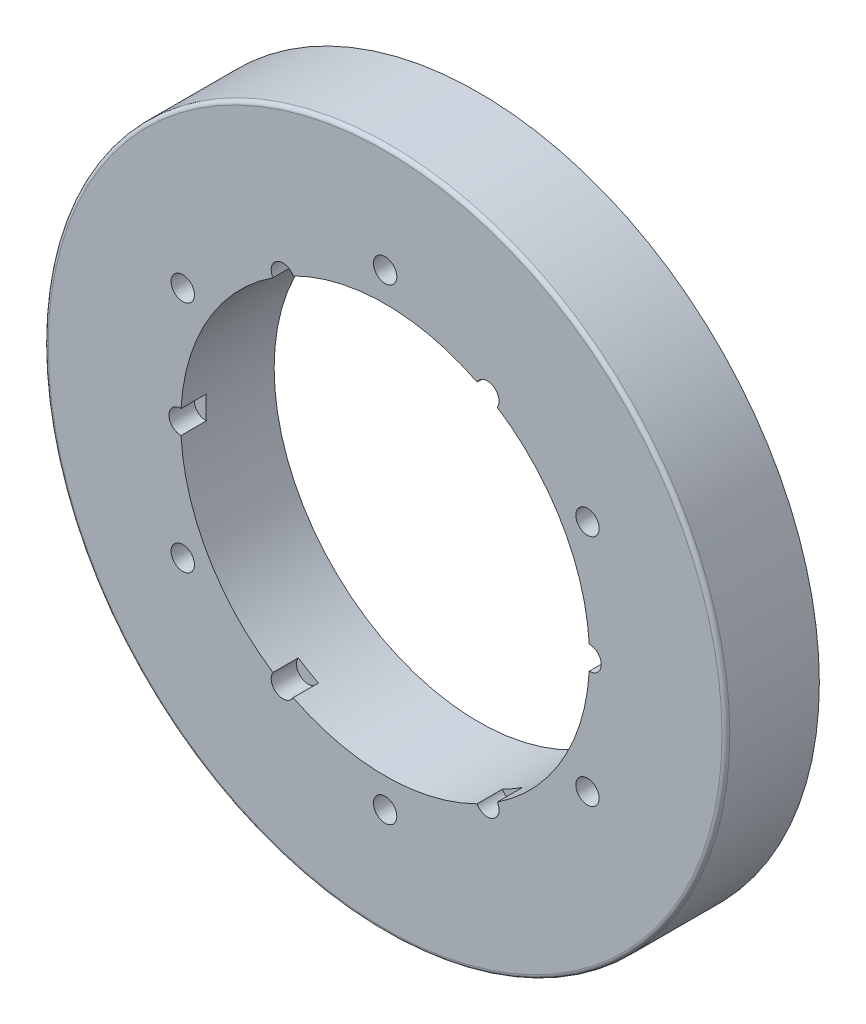
SolidWorks part; units mm, degrees
ref_plane "Front Plane" through (0, 0, 0) normal (0, 0, 1) x (1, 0, 0)
ref_plane "Top Plane" through (0, 0, 0) normal (0, 1, 0) x (1, 0, 0)
ref_plane "Right Plane" through (0, 0, 0) normal (1, 0, 0) x (0, 0, -1)
other "Configuration Table"
ref_plane "Plane1" through (0, 953.2489, 0) normal (0, 1, 0) x (1, 0, 0)
sketch "Sketch1" plane through (0, 953.2489, 0) normal (0, 1, 0) x (1, 0, 0)
  line L0 (440.0769, -691.1067) -> (265.0769, -691.1067)
  line L1 (265.0769, -691.1067) -> (265.0769, -739.1067)
  line L2 (265.0769, -739.1067) -> (438.0769, -739.1067)
  line L3 (440.0769, -737.1067) -> (440.0769, -691.1067)
  line L4 (265.0769, -691.1067) -> (265.0769, -739.1067) construction
  arc A0 (438.0769, -739.1067) -> (440.0769, -737.1067) centre (438.0769, -737.1067) ccw
revolve "Revolve1" add sketch "Sketch1" angle 360 about L4
hole_wizard "M14 Clearance Hole1" positions "Sketch3" profile "Sketch2" hole size "M14" standard "ANSI Metric"
sketch "Sketch3" plane through (0, 0, 691.1067) normal (0, 0, -1) x (-1, 0, 0)
  point P0 (-123.0487, 1035.2489)
  point P1 (-123.0487, 871.2489)
  point P2 (-265.0769, 789.2489)
  point P3 (-407.1051, 871.2489)
  point P4 (-407.1051, 1035.2489)
  point P5 (-265.0769, 1117.2489)
sketch "Sketch2" plane through (123.0487, 1035.2489, 691.1067) normal (1, 0, 0) x (0, 1, 0)
  line L0 (0, 0) -> (0, 28)
  line L1 (0, 28) -> (8.2, 28)
  line L2 (8.2, 28) -> (8.2, 0)
  line L5 (8.2, 0) -> (0, 0)
  line L10 (0, 28) -> (-8.2, 28) construction
  line L11 (0, -6.35) -> (0, 107.95) construction
  dimension "孔直径" = 16.4
  dimension "孔深度" = 28
  dimension "导头角度" = 180
hole_wizard "Ø12.0 (12) Diameter Hole1" positions "Sketch5" profile "Sketch4" hole size "Ø12.0" standard "ANSI Metric"
sketch "Sketch5" plane through (0, 0, 739.1067) normal (0, 0, 1) x (1, 0, 0)
  point P0 (370.0769, 953.2489)
  point P1 (317.5769, 1044.1816)
  point P2 (160.0769, 953.2489)
  point P3 (212.5769, 862.3163)
  point P4 (317.5769, 862.3163)
  point P5 (212.5769, 1044.1816)
  point P6 (265.0769, 833.2489)
  point P7 (161.1538, 893.2489)
  point P8 (161.1538, 1013.2489)
  point P9 (265.0769, 1073.2489)
  point P10 (368.9999, 1013.2489)
  point P11 (368.9999, 893.2489)
sketch "Sketch4" plane through (370.0769, 953.2489, 739.1067) normal (1, 0, 0) x (0, -1, 0)
  line L0 (0, 0) -> (0, 13)
  line L1 (0, 13) -> (6, 13)
  line L2 (6, 13) -> (6, 0)
  line L5 (6, 0) -> (0, 0)
  line L10 (0, 13) -> (-6, 13) construction
  line L11 (0, -6.35) -> (0, 107.95) construction
  dimension "孔直径" = 12
  dimension "孔深度" = 13
  dimension "导头角度" = 180
hole_wizard "Hole1" positions "Sketch7" profile "Sketch6" legacy
sketch "Sketch7" plane through (0, 0, 691.1067) normal (0, 0, -1) x (-1, 0, 0)
  point P0 (-265.0769, 953.2489)
sketch "Sketch6" plane through (265.0769, 953.2489, 691.1067) normal (1, 0, 0) x (0, 1, 0)
  line L0 (0, 0) -> (0, 48)
  line L1 (0, 48) -> (105, 48)
  line L2 (105, 48) -> (105, 0)
  line L3 (105, 0) -> (0, 0)
  line L4 (0, 110) -> (0, -10) construction
  dimension "直径" = 210
  dimension "深度" = 48
